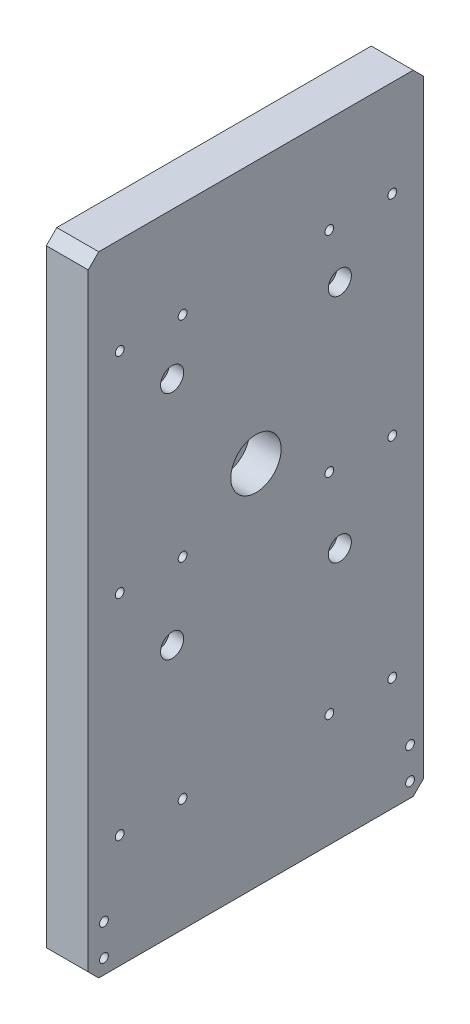
from build123d import *

# Parameters (mm, degrees)
SKETCH_1_W                = 160
SKETCH_1_H                = 300
EXTRUDE_1_DEPTH           = 20
HOLE_WIZARD_1_D           = 15.5
HOLE_WIZARD_1_DEPTH       = 25
HOLE_WIZARD_1_CBORE_D     = 24
HOLE_WIZARD_1_CBORE_DEPTH = 15
HOLE_WIZARD_1_TIP         = 4.656669797
CHAMFER_1_SIZE            = 5
HOLE_WIZARD_0_D           = 6.6
HOLE_WIZARD_0_DEPTH       = 25
HOLE_WIZARD_0_CBORE_D     = 11
HOLE_WIZARD_0_CBORE_DEPTH = 6.8
HOLE_WIZARD_0_TIP         = 1.982840043
SKETCH_6_R                = 8.1
SKETCH_6_R_2              = 10
CUT_EXTRUDE_1_DEPTH       = 2
HOLE_WIZARD_M5_1_D        = 4.2
HOLE_WIZARD_M5_1_DEPTH    = 20
HOLE_WIZARD_M5_1_TIP      = 1.2618073
HOLE_WIZARD_M5_2_D        = 4.2
HOLE_WIZARD_M5_2_DEPTH    = 20
HOLE_WIZARD_M5_2_TIP      = 1.2618073
HOLE_WIZARD_M5_3_D        = 4.2
HOLE_WIZARD_M5_3_DEPTH    = 25
HOLE_WIZARD_M5_3_TIP      = 1.2618073


with BuildPart() as part:
    # 草图1 → 凸台-拉伸1 (new body)
    with BuildSketch(Plane(origin=(0, 0, 0), x_dir=(0, 0, -1), z_dir=(1, 0, 0))):
        Rectangle(SKETCH_1_W, SKETCH_1_H)
    extrude(amount=EXTRUDE_1_DEPTH)

    # 打孔尺寸(%根据)内六角圆柱头螺钉的类型1
    with Locations(Plane(origin=(20, 0, 0), x_dir=(0, 0, -1), z_dir=(1, 0, 0))):
        with Locations((0, 25)):
            CounterBoreHole(HOLE_WIZARD_1_D / 2, HOLE_WIZARD_1_CBORE_D / 2, HOLE_WIZARD_1_CBORE_DEPTH, depth=HOLE_WIZARD_1_DEPTH)
            with Locations((0, 0, -(HOLE_WIZARD_1_DEPTH + HOLE_WIZARD_1_TIP / 2))):  # 118° drill point
                Cone(0, HOLE_WIZARD_1_D / 2, HOLE_WIZARD_1_TIP, mode=Mode.SUBTRACT)

    # 倒角1
    chamfer_1_edges = [part.edges().sort_by_distance(p)[0] for p in [
        (10, -150, -80),
        (10, -150, 80),
        (10, 150, 80),
        (10, 150, -80),
    ]]
    chamfer(chamfer_1_edges, length=CHAMFER_1_SIZE)

    # 打孔尺寸(%根据)内六角圆柱头螺钉的类型0
    with Locations(Plane(origin=(20, 0, 0), x_dir=(0, 0, -1), z_dir=(1, 0, 0))):
        with Locations((40, -30), (40, 80), (-40, -30), (-40, 80)):
            CounterBoreHole(HOLE_WIZARD_0_D / 2, HOLE_WIZARD_0_CBORE_D / 2, HOLE_WIZARD_0_CBORE_DEPTH, depth=HOLE_WIZARD_0_DEPTH)
            with Locations((0, 0, -(HOLE_WIZARD_0_DEPTH + HOLE_WIZARD_0_TIP / 2))):  # 118° drill point
                Cone(0, HOLE_WIZARD_0_D / 2, HOLE_WIZARD_0_TIP, mode=Mode.SUBTRACT)

    # 草图6 → 切除-拉伸1 (cut)
    with BuildSketch(Plane.ZY):
        with Locations((-40, 80)):
            Circle(SKETCH_6_R)
        with Locations((-40, -30)):
            Circle(SKETCH_6_R)
        with Locations((0, 25)):
            Circle(SKETCH_6_R_2)
        with Locations((40, -30)):
            Circle(SKETCH_6_R)
        with Locations((40, 80)):
            Circle(SKETCH_6_R)
    extrude(amount=-CUT_EXTRUDE_1_DEPTH, mode=Mode.SUBTRACT)

    # M5 螺纹孔1
    with Locations(Plane.ZY):
        with Locations((65, -96), (35, -96), (65, 4), (35, 4), (65, 104), (35, 104), (-35, 104), (-65, 104), (-35, 4), (-65, 4), (-35, -96), (-65, -96)):
            Hole(HOLE_WIZARD_M5_1_D / 2, depth=HOLE_WIZARD_M5_1_DEPTH)
            with Locations((0, 0, -(HOLE_WIZARD_M5_1_DEPTH + HOLE_WIZARD_M5_1_TIP / 2))):  # 118° drill point
                Cone(0, HOLE_WIZARD_M5_1_D / 2, HOLE_WIZARD_M5_1_TIP, mode=Mode.SUBTRACT)

    # M5 螺纹孔2
    with Locations(Plane.ZY):
        with Locations((72.5, -143), (72.5, -128)):
            Hole(HOLE_WIZARD_M5_2_D / 2, depth=HOLE_WIZARD_M5_2_DEPTH)
            with Locations((0, 0, -(HOLE_WIZARD_M5_2_DEPTH + HOLE_WIZARD_M5_2_TIP / 2))):  # 118° drill point
                Cone(0, HOLE_WIZARD_M5_2_D / 2, HOLE_WIZARD_M5_2_TIP, mode=Mode.SUBTRACT)

    # M5 螺纹孔3
    with Locations(Plane.ZY):
        with Locations((-73.5, -143), (-73.5, -128)):
            Hole(HOLE_WIZARD_M5_3_D / 2, depth=HOLE_WIZARD_M5_3_DEPTH)
            with Locations((0, 0, -(HOLE_WIZARD_M5_3_DEPTH + HOLE_WIZARD_M5_3_TIP / 2))):  # 118° drill point
                Cone(0, HOLE_WIZARD_M5_3_D / 2, HOLE_WIZARD_M5_3_TIP, mode=Mode.SUBTRACT)


solid = part.part
